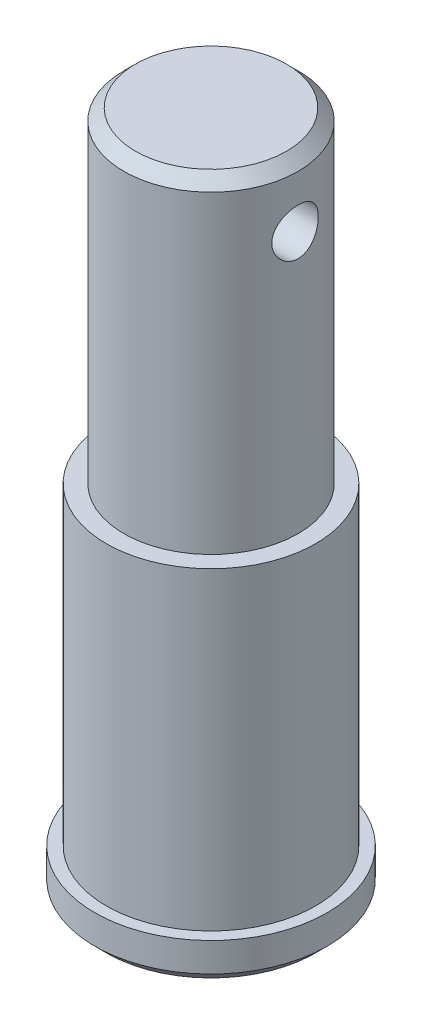
SolidWorks part; units mm, degrees
ref_plane "前视基准面" through (0, 0, 0) normal (0, 0, 1) x (1, 0, 0)
ref_plane "上视基准面" through (0, 0, 0) normal (0, 1, 0) x (1, 0, 0)
ref_plane "右视基准面" through (0, 0, 0) normal (1, 0, 0) x (0, 0, -1)
sketch "草图1" plane through (0, 0, 0) normal (0, 0, 1) x (1, 0, 0)
  line L0 (0, 29.25) -> (0, -29.25)
  line L1 (0, -29.25) -> (10, -29.25)
  line L2 (10, -29.25) -> (10, -25.75)
  line L4 (7.5, 1.25) -> (7.5, 29.25)
  line L5 (7.5, 29.25) -> (0, 29.25)
  line L6 (7.5, 1.25) -> (9, 1.25)
  line L7 (9, 1.25) -> (9, -25.75)
  line L8 (9, -25.75) -> (10, -25.75)
  point P4 (0, 0)
  dimension "D1" = 58.5
  dimension "D2" = 7.5
  dimension "D3" = 9
  dimension "D4" = 10
  dimension "D5" = 27
  dimension "D6" = 3.5
revolve "旋转1" add sketch "草图1" angle 360 about L0
sketch "草图2" plane through (0, 0, 0) normal (1, 0, 0) x (0, 0, -1)
  line L0 (7.5, 29.25) -> (-7.5, 29.25) construction
  circle A0 centre (0, 23.75) radius 2
  dimension "D1" = 4
  dimension "D2" = 5.5
extrude "切除-拉伸1" cut sketch "草图2" against normal mid plane 20
chamfer "倒角1" distance 1 angle 45 2 edges at (-7.5, 29.25, 0) (-10, -29.25, 0)
